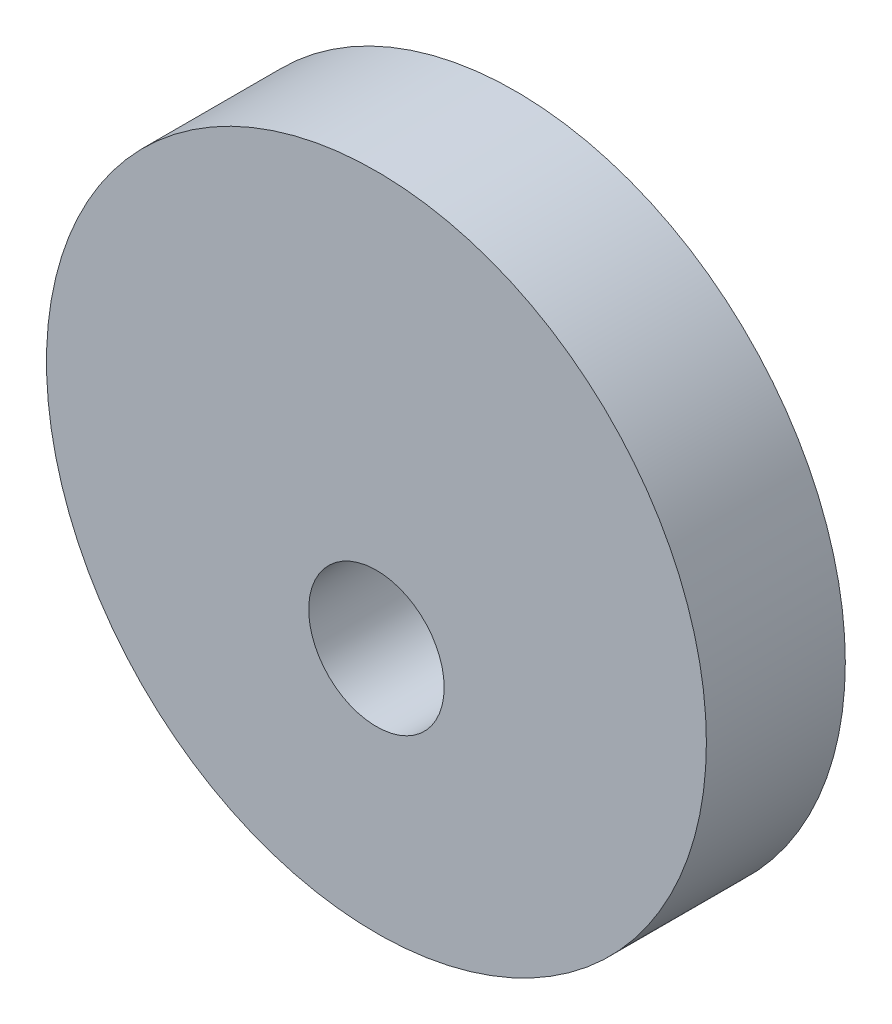
SolidWorks part; units mm, degrees
ref_plane "Front Plane" through (0, 0, 0) normal (0, 0, 1) x (1, 0, 0)
ref_plane "Top Plane" through (0, 0, 0) normal (0, 1, 0) x (1, 0, 0)
ref_plane "Right Plane" through (0, 0, 0) normal (1, 0, 0) x (0, 0, -1)
sketch "Sketch1" plane through (0, 0, 0) normal (0, 0, 1) x (1, 0, 0)
  line L0 (0, -74.77) -> (0, -69.97) construction
  line L1 (0, -50.97) -> (0, -69.97) construction
  line L2 (0, -74.77) -> (9.6168, -74.77) construction
  circle A0 centre (0, -69.97) radius 19
  circle A1 centre (0, -74.77) radius 3.9 construction
  circle A2 centre (0, -74.77) radius 3.9
  dimension "D1" = 38
  dimension "D3" = 4.8
extrude "Boss-Extrude1" add sketch "Sketch1" along normal mid plane 8
sketch "Sketch3" plane through (0, 0, -4) normal (0, 0, -1) x (-1, 0, 0)
  line L0 (-1.8494, -51.0602) -> (-1.517, -51.6741)
  line L1 (-45.0623, -65.0545) -> (-16.4931, -117.8162) construction
  circle A0 centre (0, -69.97) radius 19 construction
